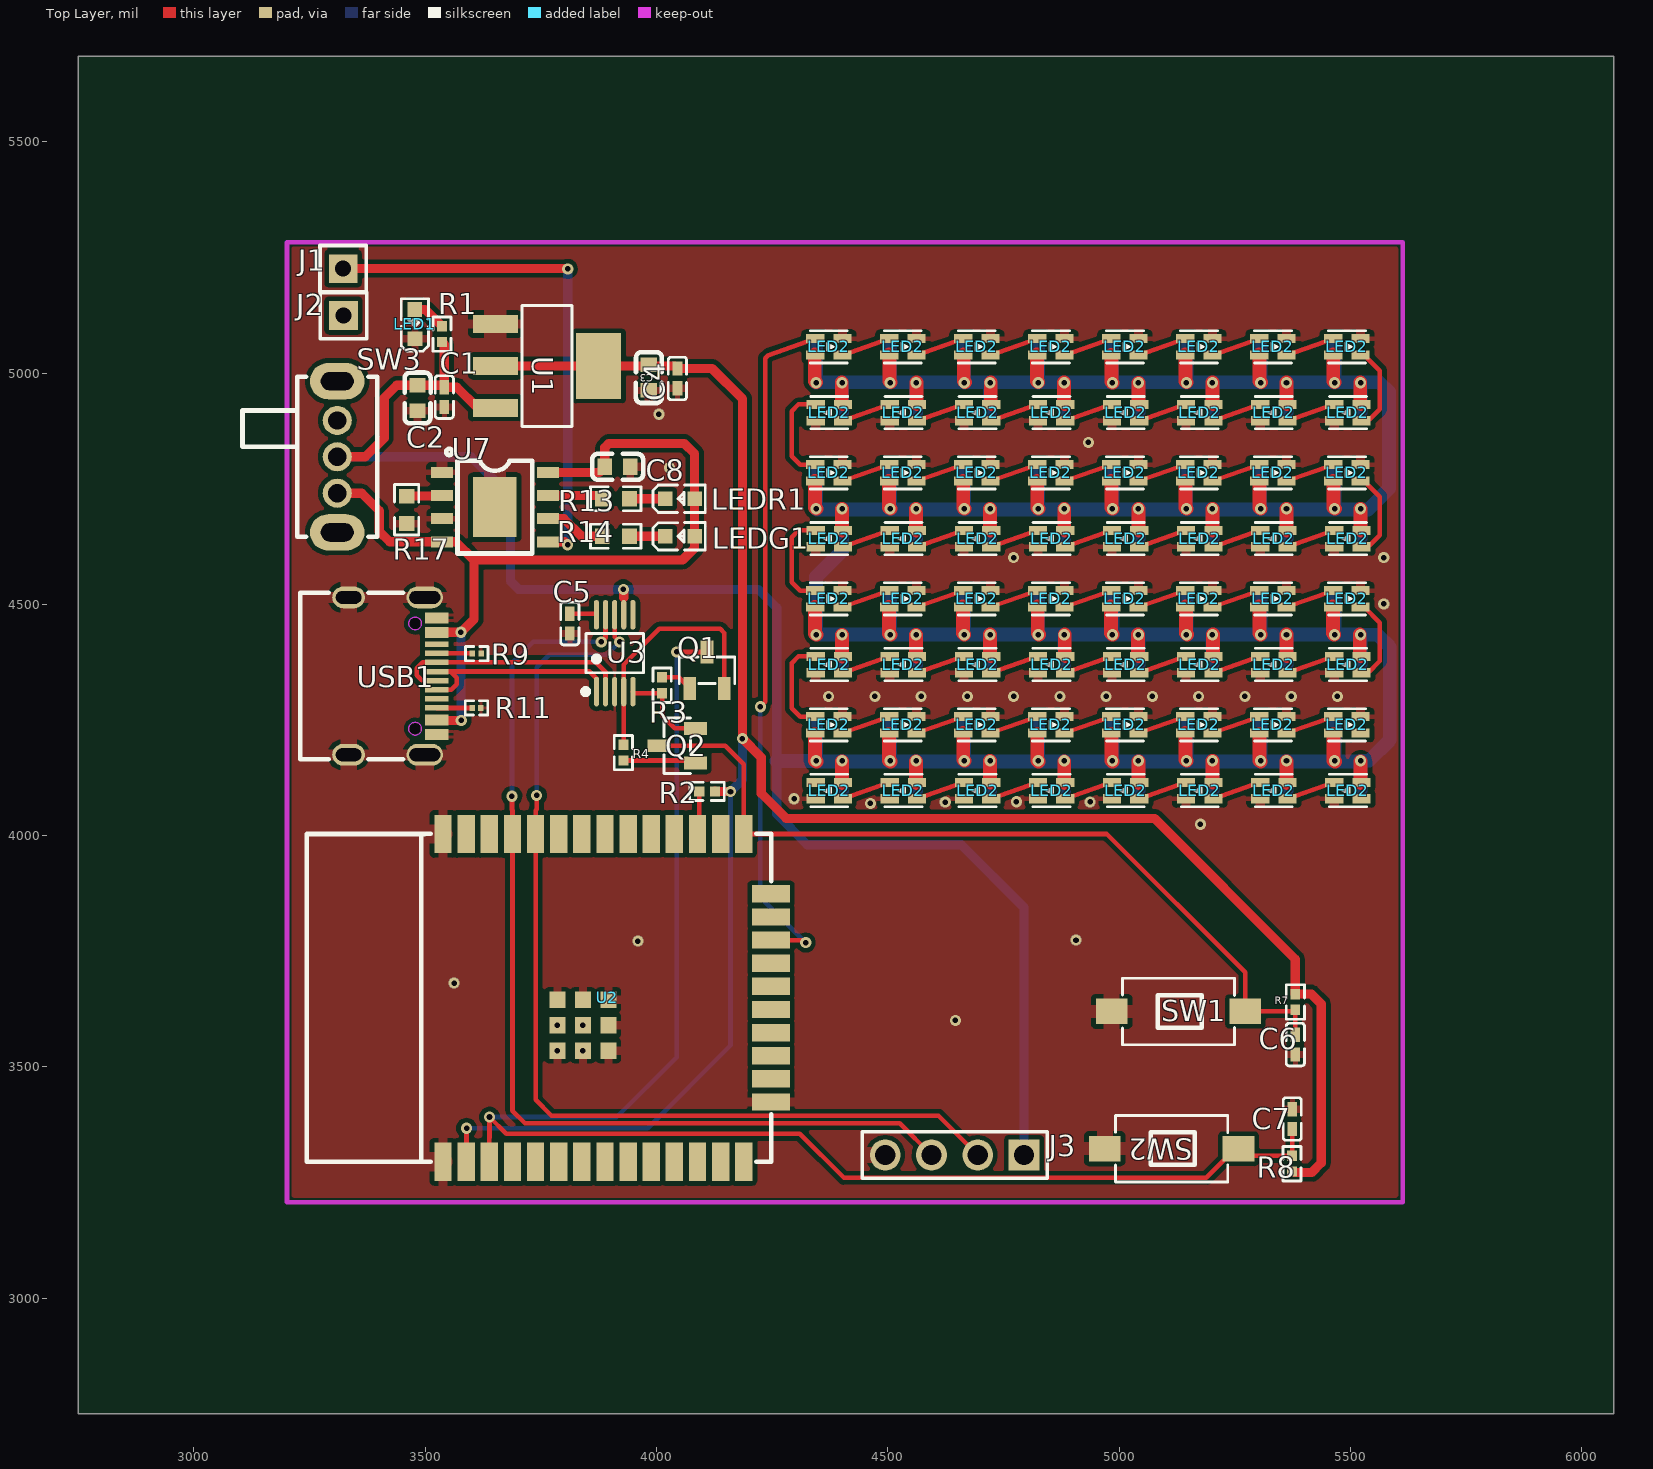
[diagram p0: Top Layer view]
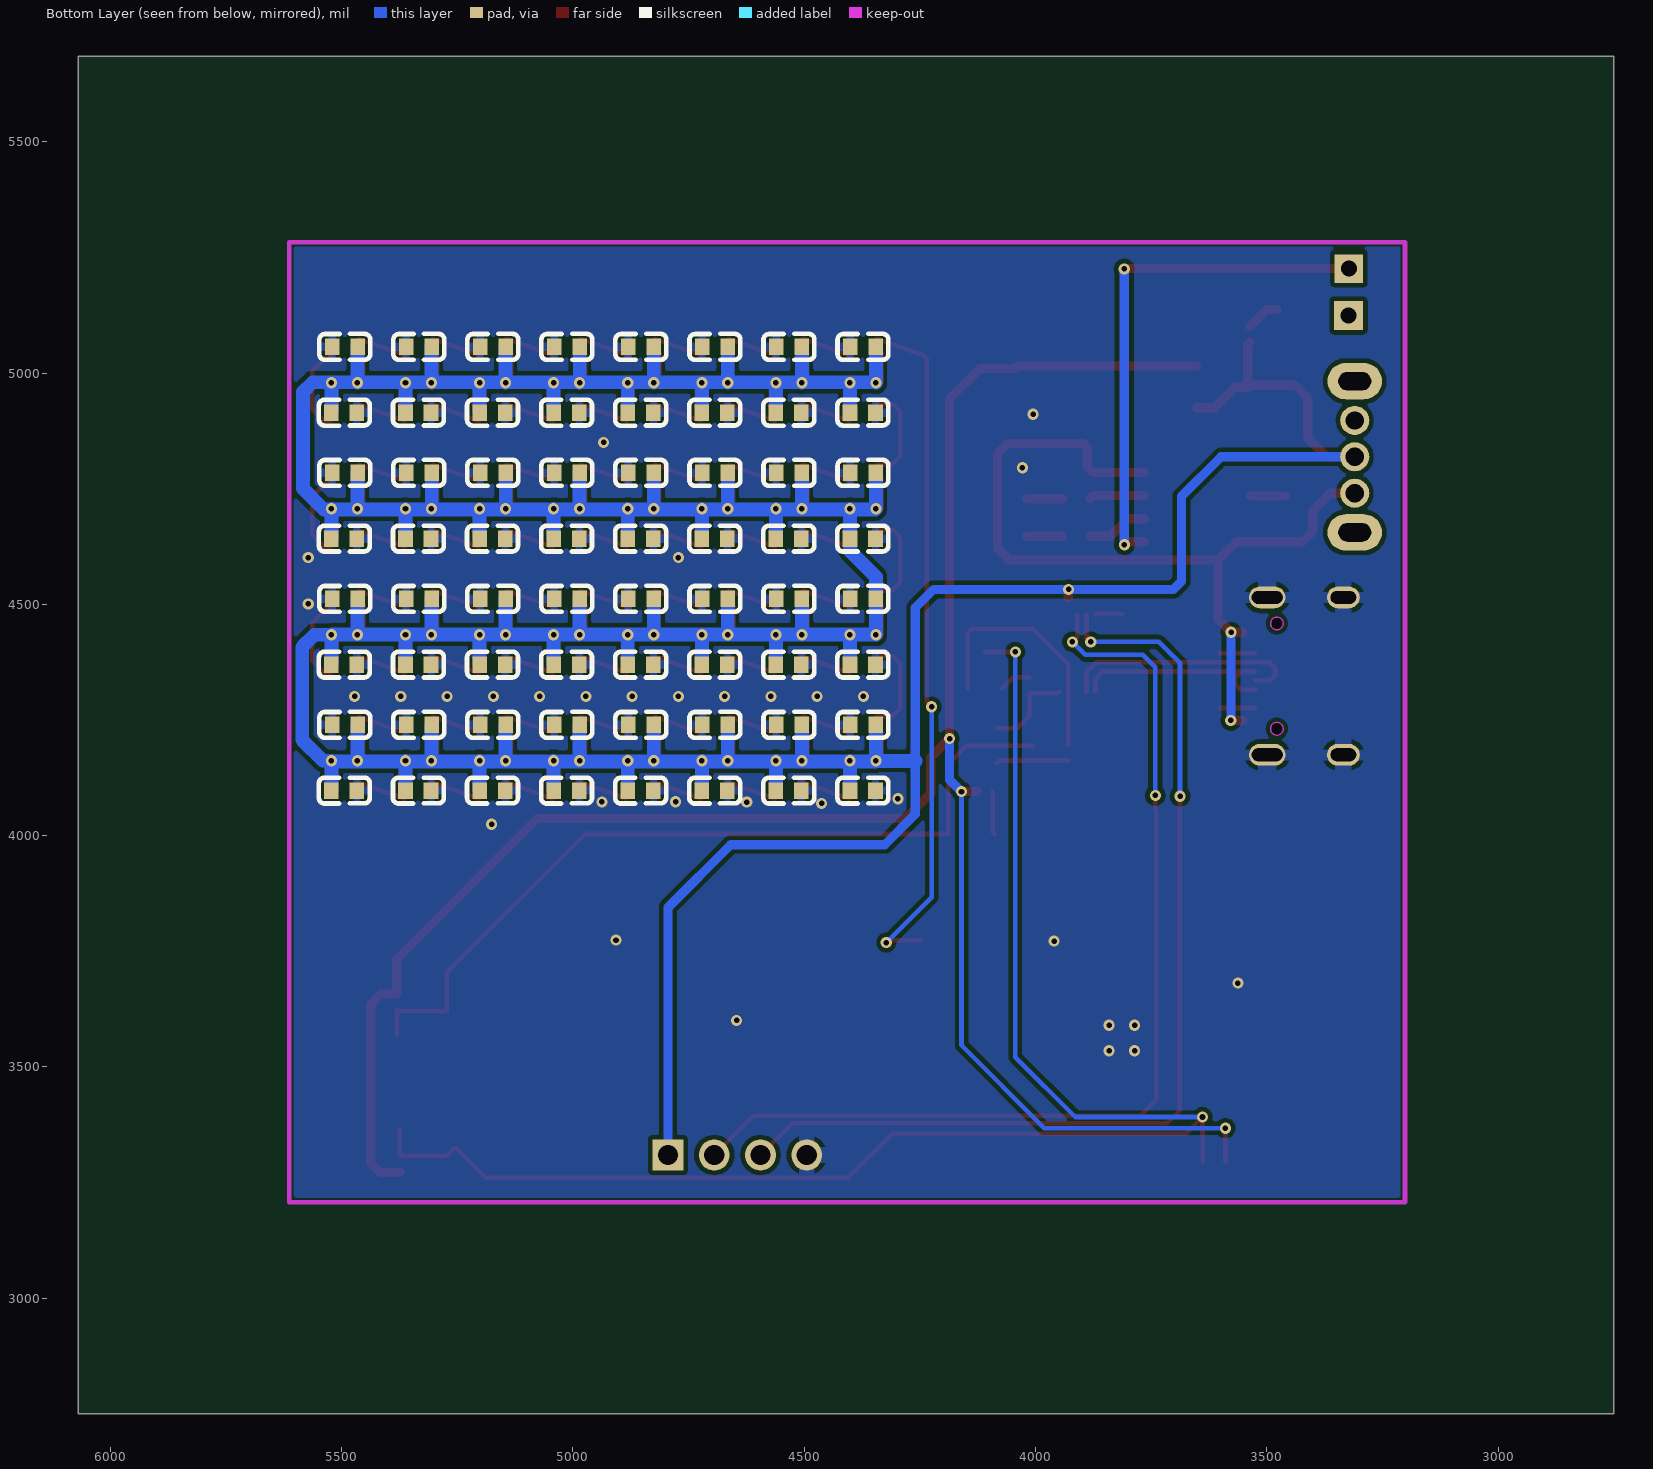
[diagram p1: Bottom Layer view, seen from below]
# Altium PCB MISC52063.pcbdoc
Units mil, origin at the board's own origin, x right, y up, seen from the top; angles counter-clockwise.
Board outline 3318.73 x 2934.56 mil, 2 copper layers (Top Layer, Bottom Layer), stack 62.206 mil thick; 99 components, 49 nets, 539 pads, 112 vias.

## Layer stack, top to bottom
Top Solder Mask Layer: solder mask 0.394, Dk 3.3
Top Layer: signal copper 1.379
Dielectric1: surface 59.449, FR4, Dk 4.5
Bottom Layer: signal copper 1.378
Bottom Solder Mask Layer: solder mask 0.394, Dk 3.3

## Board outline
6068.73,2750 2750,2750 2750,5684.56 6068.73,5684.56

## Design rules (kind name [scope] priority, off if disabled: settings)
BoardOutlineClearance Plane_Default_1 [All] p2 off: genericclearance=5.98 ignorepadtopadclearanceinfootprint=FALSE except(0: Arc-SplitContinuation Track-SplitContinuation SMDPad-SplitContinuation THPad-SplitContinuation Via-SplitContinuation Fill-SplitContinuation Region-SplitContinuation Poly-SplitContinuation Text-SplitContinuation Hole-SplitContinuation; 5.98: Arc-OutlineEdge Track-OutlineEdge SMDPad-OutlineEdge THPad-OutlineEdge Via-OutlineEdge Fill-OutlineEdge Region-OutlineEdge Poly-OutlineEdge Text-OutlineEdge Hole-OutlineEdge Arc-CutoutEdge Track-CutoutEdge SMDPad-CutoutEdge THPad-CutoutEdge Via-CutoutEdge Fill-CutoutEdge Region-CutoutEdge Poly-CutoutEdge Text-CutoutEdge Hole-CutoutEdge)
BoardOutlineClearance Copper_gge30915_1 [All] p4 off: genericclearance=5.98 ignorepadtopadclearanceinfootprint=FALSE except(0: Arc-SplitContinuation Track-SplitContinuation SMDPad-SplitContinuation THPad-SplitContinuation Via-SplitContinuation Fill-SplitContinuation Region-SplitContinuation Poly-SplitContinuation Text-SplitContinuation Hole-SplitContinuation; 5.98: Arc-OutlineEdge Track-OutlineEdge SMDPad-OutlineEdge THPad-OutlineEdge Via-OutlineEdge Fill-OutlineEdge Region-OutlineEdge Text-OutlineEdge Hole-OutlineEdge Arc-CutoutEdge Track-CutoutEdge SMDPad-CutoutEdge THPad-CutoutEdge Via-CutoutEdge Fill-CutoutEdge Region-CutoutEdge Text-CutoutEdge Hole-CutoutEdge; 10: Poly-OutlineEdge Poly-CutoutEdge)
BoardOutlineClearance Copper_gge30960_1 [All] p6 off: genericclearance=5.98 ignorepadtopadclearanceinfootprint=FALSE except(0: Arc-SplitContinuation Track-SplitContinuation SMDPad-SplitContinuation THPad-SplitContinuation Via-SplitContinuation Fill-SplitContinuation Region-SplitContinuation Poly-SplitContinuation Text-SplitContinuation Hole-SplitContinuation; 5.98: Arc-OutlineEdge Track-OutlineEdge SMDPad-OutlineEdge THPad-OutlineEdge Via-OutlineEdge Fill-OutlineEdge Region-OutlineEdge Text-OutlineEdge Hole-OutlineEdge Arc-CutoutEdge Track-CutoutEdge SMDPad-CutoutEdge THPad-CutoutEdge Via-CutoutEdge Fill-CutoutEdge Region-CutoutEdge Text-CutoutEdge Hole-CutoutEdge; 10: Poly-OutlineEdge Poly-CutoutEdge)
BoardOutlineClearance Default_1 [All] p8: genericclearance=5.98 ignorepadtopadclearanceinfootprint=FALSE except(0: Arc-SplitContinuation Track-SplitContinuation SMDPad-SplitContinuation THPad-SplitContinuation Via-SplitContinuation Fill-SplitContinuation Region-SplitContinuation Poly-SplitContinuation Text-SplitContinuation Hole-SplitContinuation; 5.98: Arc-OutlineEdge Track-OutlineEdge SMDPad-OutlineEdge THPad-OutlineEdge Via-OutlineEdge Fill-OutlineEdge Region-OutlineEdge Text-OutlineEdge Hole-OutlineEdge Arc-CutoutEdge Track-CutoutEdge SMDPad-CutoutEdge THPad-CutoutEdge Via-CutoutEdge Fill-CutoutEdge Region-CutoutEdge Text-CutoutEdge Hole-CutoutEdge; 10: Poly-OutlineEdge Poly-CutoutEdge)
Clearance Plane_Default [All] p1 off: gap=5.98 ignorepadtopadclearanceinfootprint=FALSE except(0: Arc-Arc)
Clearance Copper_gge30915 [All] p3 off: gap=5.98 ignorepadtopadclearanceinfootprint=FALSE except(0: Arc-Arc; 10: Poly-Track Poly-SMDPad Poly-THPad Poly-Via Poly-Fill Poly-Region Poly-Poly Poly-Arc Poly-Text Poly-Hole)
Clearance Copper_gge30960 [All] p5 off: gap=5.98 ignorepadtopadclearanceinfootprint=FALSE except(0: Arc-Arc; 10: Poly-Track Poly-SMDPad Poly-THPad Poly-Via Poly-Fill Poly-Region Poly-Poly Poly-Arc Poly-Text Poly-Hole)
Clearance Default [All] p7: gap=5.98 ignorepadtopadclearanceinfootprint=FALSE except(0: Arc-Arc; 10: Poly-Track Poly-SMDPad Poly-THPad Poly-Via Poly-Fill Poly-Region Poly-Poly Poly-Arc Poly-Text Poly-Hole)
DiffPairsRouting differentialPair [All] p1: maxlimit=6 minlimit=6 mostfreqgap=6 toplayer_minwidth=5 toplayer_prefwidth=10 toplayer_maxwidth=100 toplayer_mingap=6 toplayer_prefgap=6 toplayer_maxgap=6 bottomlayer_minwidth=5 bottomlayer_prefwidth=10 bottomlayer_maxwidth=100 bottomlayer_mingap=6 bottomlayer_prefgap=6 bottomlayer_maxgap=6 maxuncoupledlength=10
HoleToHoleClearance otherClearance [All] p1: gap=11.8 allowstackedmicrovias=TRUE
Length netLength [All] p1: minlimit=0 maxlimit=0
PasteMaskExpansion Common [All] p1: expansion=0
PlaneConnect Default_4 [All] p1: planeconnectstyle=Relief reliefexpansion=20 reliefentries=4 reliefconductorwidth=0 reliefairgap=10
PolygonConnect gge30960 [All] p1 off: connectstyle=Relief reliefconductorwidth=0 reliefentries=4 polygonreliefangle="90 Angle" airgapwidth=10 via.connectstyle=Relief via.reliefconductorwidth=10 via.reliefentries=4 via.polygonreliefangle="90 Angle" via.airgapwidth=10
PolygonConnect gge30915 [All] p2: connectstyle=Relief reliefconductorwidth=0 reliefentries=4 polygonreliefangle="90 Angle" airgapwidth=10 via.connectstyle=Relief via.reliefconductorwidth=10 via.reliefentries=4 via.polygonreliefangle="90 Angle" via.airgapwidth=10
RoutingVias Default_3 [All] p1: holewidth=12.01 width=24.02 viastyle="Through Hole" minholewidth=12.01 minwidth=24.02 maxholewidth=2362 maxwidth=3938
SolderMaskExpansion Common_1 [IsVia] p1: expansion=-1000 istentingtop=TRUE
SolderMaskExpansion Common_1 [All] p2: expansion=2 istentingtop=FALSE
Width Default_2 [All] p1: maxlimit=1000 minlimit=10 preferedwidth=10

## Components (designator, comment, footprint, x,y, rotation, side; value= is the part's Value field where it differs from the comment)
C1 "100nF" C0402 3541.1,4947.9 r90 top
C2 "22uF" C0603 3483.26,4945.73 r270 top
C3 "22uF" C0603 3983.19,4989.83 r270 top
C4 "100nF" C0402 4044.95,4988.21 r90 top
C5 "100nF" C0402 3812.38,4458.38 r90 top
C6 "100nF" C0402 5380.55,3548.42 r270 top
C7 "100nF" C0402 5373.94,3387.47 r90 top
C8 "100nF" C0603 3915.51,4797.39 r180 top
J1 "HDR-M-2.54_1x1" HDR-M-2.54_1X1 3322.44,5225.66 r90 top
J2 "HDR-M-2.54_1x1" HDR-M-2.54_1X1 3323.19,5124.2 r90 top
J3 "2.54-1*4" HDR-TH_4P-P2.54-V-M-1 4644.17,3309.76 r180 top
LED1 "XL-1608SURC-06" LED0603-RD_RED 3477.68,5105.77 r90 top
LED2 "WS2812B-0807幻彩" LED-SMD_4P-L2.0-W1.8-TL 5334.08,4097.5 r0 top
LED2 "WS2812B-0807幻彩" LED-SMD_4P-L2.0-W1.8-TL 5494.19,4097.5 r0 top
LED2 "WS2812B-0807幻彩" LED-SMD_4P-L2.0-W1.8-TL 5013.86,4097.5 r0 top
LED2 "WS2812B-0807幻彩" LED-SMD_4P-L2.0-W1.8-TL 5173.97,4097.5 r0 top
LED2 "WS2812B-0807幻彩" LED-SMD_4P-L2.0-W1.8-TL 4693.64,4097.5 r0 top
LED2 "WS2812B-0807幻彩" LED-SMD_4P-L2.0-W1.8-TL 4853.75,4097.5 r0 top
LED2 "WS2812B-0807幻彩" LED-SMD_4P-L2.0-W1.8-TL 4533.53,4097.5 r0 top
LED2 "WS2812B-0807幻彩" LED-SMD_4P-L2.0-W1.8-TL 5012.21,4239.55 r180 top
LED2 "WS2812B-0807幻彩" LED-SMD_4P-L2.0-W1.8-TL 5332.2,4239.55 r180 top
LED2 "WS2812B-0807幻彩" LED-SMD_4P-L2.0-W1.8-TL 4852.21,4239.55 r180 top
LED2 "WS2812B-0807幻彩" LED-SMD_4P-L2.0-W1.8-TL 5492.2,4239.55 r180 top
LED2 "WS2812B-0807幻彩" LED-SMD_4P-L2.0-W1.8-TL 5172.21,4239.55 r180 top
LED2 "WS2812B-0807幻彩" LED-SMD_4P-L2.0-W1.8-TL 4532.21,4239.55 r180 top
LED2 "WS2812B-0807幻彩" LED-SMD_4P-L2.0-W1.8-TL 4692.21,4239.55 r180 top
LED2 "WS2812B-0807幻彩" LED-SMD_4P-L2.0-W1.8-TL 4853.75,4369.81 r0 top
LED2 "WS2812B-0807幻彩" LED-SMD_4P-L2.0-W1.8-TL 4533.53,4369.81 r0 top
LED2 "WS2812B-0807幻彩" LED-SMD_4P-L2.0-W1.8-TL 5494.19,4369.81 r0 top
LED2 "WS2812B-0807幻彩" LED-SMD_4P-L2.0-W1.8-TL 5334.08,4369.81 r0 top
LED2 "WS2812B-0807幻彩" LED-SMD_4P-L2.0-W1.8-TL 5013.86,4369.81 r0 top
LED2 "WS2812B-0807幻彩" LED-SMD_4P-L2.0-W1.8-TL 5173.97,4369.81 r0 top
LED2 "WS2812B-0807幻彩" LED-SMD_4P-L2.0-W1.8-TL 4693.64,4369.81 r0 top
LED2 "WS2812B-0807幻彩" LED-SMD_4P-L2.0-W1.8-TL 5332.2,4784.17 r180 top
LED2 "WS2812B-0807幻彩" LED-SMD_4P-L2.0-W1.8-TL 5012.21,4784.17 r180 top
LED2 "WS2812B-0807幻彩" LED-SMD_4P-L2.0-W1.8-TL 5172.21,4784.17 r180 top
LED2 "WS2812B-0807幻彩" LED-SMD_4P-L2.0-W1.8-TL 4692.21,4784.17 r180 top
LED2 "WS2812B-0807幻彩" LED-SMD_4P-L2.0-W1.8-TL 4532.21,4784.17 r180 top
LED2 "WS2812B-0807幻彩" LED-SMD_4P-L2.0-W1.8-TL 5492.2,4784.17 r180 top
LED2 "WS2812B-0807幻彩" LED-SMD_4P-L2.0-W1.8-TL 4852.21,4784.17 r180 top
LED2 "WS2812B-0807幻彩" LED-SMD_4P-L2.0-W1.8-TL 5494.19,4642.11 r0 top
LED2 "WS2812B-0807幻彩" LED-SMD_4P-L2.0-W1.8-TL 5334.08,4642.11 r0 top
LED2 "WS2812B-0807幻彩" LED-SMD_4P-L2.0-W1.8-TL 4532.21,5056.47 r180 top
LED2 "WS2812B-0807幻彩" LED-SMD_4P-L2.0-W1.8-TL 5332.2,5056.47 r180 top
LED2 "WS2812B-0807幻彩" LED-SMD_4P-L2.0-W1.8-TL 5012.21,5056.47 r180 top
LED2 "WS2812B-0807幻彩" LED-SMD_4P-L2.0-W1.8-TL 5172.21,5056.47 r180 top
LED2 "WS2812B-0807幻彩" LED-SMD_4P-L2.0-W1.8-TL 4692.21,5056.47 r180 top
LED2 "WS2812B-0807幻彩" LED-SMD_4P-L2.0-W1.8-TL 4852.21,5056.47 r180 top
LED2 "WS2812B-0807幻彩" LED-SMD_4P-L2.0-W1.8-TL 5494.19,4914.42 r0 top
LED2 "WS2812B-0807幻彩" LED-SMD_4P-L2.0-W1.8-TL 4533.53,4914.42 r0 top
LED2 "WS2812B-0807幻彩" LED-SMD_4P-L2.0-W1.8-TL 5334.08,4914.42 r0 top
LED2 "WS2812B-0807幻彩" LED-SMD_4P-L2.0-W1.8-TL 4853.75,4914.42 r0 top
LED2 "WS2812B-0807幻彩" LED-SMD_4P-L2.0-W1.8-TL 4693.64,4914.42 r0 top
LED2 "WS2812B-0807幻彩" LED-SMD_4P-L2.0-W1.8-TL 5173.97,4914.42 r0 top
LED2 "WS2812B-0807幻彩" LED-SMD_4P-L2.0-W1.8-TL 5013.86,4914.42 r0 top
LED2 "WS2812B-0807幻彩" LED-SMD_4P-L2.0-W1.8-TL 4853.75,4642.11 r0 top
LED2 "WS2812B-0807幻彩" LED-SMD_4P-L2.0-W1.8-TL 4533.53,4642.11 r0 top
LED2 "WS2812B-0807幻彩" LED-SMD_4P-L2.0-W1.8-TL 5013.86,4642.11 r0 top
LED2 "WS2812B-0807幻彩" LED-SMD_4P-L2.0-W1.8-TL 4693.64,4642.11 r0 top
LED2 "WS2812B-0807幻彩" LED-SMD_4P-L2.0-W1.8-TL 5492.2,4511.86 r180 top
LED2 "WS2812B-0807幻彩" LED-SMD_4P-L2.0-W1.8-TL 5012.21,4511.86 r180 top
LED2 "WS2812B-0807幻彩" LED-SMD_4P-L2.0-W1.8-TL 5332.2,4511.86 r180 top
LED2 "WS2812B-0807幻彩" LED-SMD_4P-L2.0-W1.8-TL 4852.21,4511.86 r180 top
LED2 "WS2812B-0807幻彩" LED-SMD_4P-L2.0-W1.8-TL 5172.21,4511.86 r180 top
LED2 "WS2812B-0807幻彩" LED-SMD_4P-L2.0-W1.8-TL 4532.21,4511.86 r180 top
LED2 "WS2812B-0807幻彩" LED-SMD_4P-L2.0-W1.8-TL 4692.21,4511.86 r180 top
LED2 "WS2812B-0807幻彩" LED-SMD_4P-L2.0-W1.8-TL 5492.2,5056.47 r180 top
LED2 "WS2812B-0807幻彩" LED-SMD_4P-L2.0-W1.8-TL 5173.97,4642.11 r0 top
LED2 "WS2812B-0807幻彩" LED-SMD_4P-L2.0-W1.8-TL 4373.42,4642.11 r0 top
LED2 "WS2812B-0807幻彩" LED-SMD_4P-L2.0-W1.8-TL 4373.42,4369.81 r0 top
LED2 "WS2812B-0807幻彩" LED-SMD_4P-L2.0-W1.8-TL 4373.42,4914.42 r0 top
LED2 "WS2812B-0807幻彩" LED-SMD_4P-L2.0-W1.8-TL 4373.42,4097.5 r0 top
LED2 "WS2812B-0807幻彩" LED-SMD_4P-L2.0-W1.8-TL 4372.21,5056.47 r180 top
LED2 "WS2812B-0807幻彩" LED-SMD_4P-L2.0-W1.8-TL 4372.21,4239.55 r180 top
LED2 "WS2812B-0807幻彩" LED-SMD_4P-L2.0-W1.8-TL 4372.21,4784.17 r180 top
LED2 "WS2812B-0807幻彩" LED-SMD_4P-L2.0-W1.8-TL 4372.21,4511.86 r180 top
LEDG1 "" LED_0603 4052.62,4647.17 r0 top
LEDR1 "" LED_0603 4052.62,4728.32 r0 top
Q1 "SS8050-G" SOT-23-3_L2.9-W1.3-P1.90-LS2.4-BR 4108.98,4357.55 r270 top
Q2 "SS8050-G" SOT-23-3_L2.9-W1.3-P1.90-LS2.4-BR 4044.49,4194.4 r0 top
R1 "2kΩ" R0402 3536.18,5084.08 r270 top
R2 "10kΩ" R0402 4108.98,4095.74 r0 top
R3 "10kΩ" R0402 4011.97,4325.03 r90 top
R4 "10kΩ" R0402 3928.14,4179.47 r270 top
R7 "10kΩ" R0402 5380.55,3640.46 r270 top
R8 "10kΩ" R0402 5373.39,3291.02 r90 top
R9 "5.1kΩ" R0201 3611.31,4393.38 r180 top
R11 "5.1kΩ" R0201 3610.75,4275.98 r0 top
R13 "1K" R0603 3911.86,4728.32 r0 top
R14 "1K" R0603 3911.86,4647.17 r0 top
R17 "1.2K" R0603 3459.69,4704.24 r90 top
SW1 "TSB008A2530A" SW-SMD_L6.0-W3.5-LS8.0 5128.11,3620.07 r0 top
SW2 "TSB008A2530A" SW-SMD_L6.0-W3.5-LS8.0 5113.23,3323.54 r0 top
SW3 "" 拨动开关_侧 3309.76,4818.89 r270 top
U1 "AMS1117-3.3" SOT-223-4_L6.5-W3.5-P2.30-LS7.0-BR 3763.26,5015.18 r180 top
U2 "ESP32-WROOM-32E-N16" WIFI-SMD_ESP32-WROOM-32E 3892.87,3649.29 r0 top
U3 "CH340E" MSOP-10_L3.0-W3.0-P0.50-LS5.0-BL 3909.35,4394.48 r0 top
U7 "TP4056" ESOP-8_L4.9-W3.9-P1.27-LS6.0-BL-EP 3650.42,4710.13 r270 top
USB1 "KH-TYPE-C-16P-T" USB-C-SMD_KH-TYPE-C-16P 3429.41,4344.87 r270 top

## Footprints (in the part's own frame and the unit in brackets; to place one, negate y for a bottom-side part, rotate by r counter-clockwise, add the part's x,y. Pads: shape width x height; smd on the part's side, far side on the other; paste and mask are expansions set on the pad)
C0402 [mm]
  rect 0.79x0.54 smd paste-100 mask+0.051: 1(-0.545,0) 2(0.545,0)
  silkscreen extent -1.17,-0.5 1.17,0.5
C0603 [mm]
  rect 0.8x0.9 smd: 1(-0.7,0) 2(0.7,0)
  silkscreen extent -1.41,-0.71 1.39,0.72
ESOP-8_L4.9-W3.9-P1.27-LS6.0-BL-EP [mm]
  rect 0.6x1.2 smd paste+0 mask+0.051: 1(-1.905,-2.908) 2(-0.635,-2.908) 3(0.635,-2.908) 4(1.905,-2.908) 5(1.905,2.908) 6(0.635,2.908) 7(-0.635,2.908) 8(-1.905,2.908)
  rect 3.3x2.4 smd paste+0 mask+0.051: 9(0,0)
  silkscreen extent -3.2,-2.67 2.55,2.05
HDR-M-2.54_1X1 [mil]
  rect 62x62 hole 35 paste+0 mask+2: 1(0,0)
  silkscreen extent -50,-50 50,50
HDR-TH_4P-P2.54-V-M-1 [mm]
  rect 1.7x1.7 hole 1.1: 1(-3.81,0)
  round 1.7 hole 1.1: 2(-1.27,0) 3(1.27,0) 4(3.81,0)
  silkscreen extent -5.08,-1.27 5.08,1.27
LED0603-RD_RED [mm]
  rect 0.8x0.8 smd: 1(-0.8,-0.003) 2(0.8,0.003)
  silkscreen extent -1.49,-0.75 1.39,0.76
LED-SMD_4P-L2.0-W1.8-TL [mm]
  rect 1x0.5 smd paste+0 mask+0.05: 1(0.75,0.45) 2(-0.75,0.45) 3(-0.75,-0.45) 4(0.75,-0.45)
  rect 0.8x0.9 smd far side: 5(-0.705,-0.003) 6(0.695,-0.003)
  silkscreen extent -1.02,-0.89 1.02,0.89
LED_0603 [mil]
  rect 31.5x31.5 smd paste+0 mask+2: 1(-33.5,-0.4) 2(29.5,-0.2)
  silkscreen extent -61,-30 53,30
MSOP-10_L3.0-W3.0-P0.50-LS5.0-BL [mm]
  oval 0.28x1.62 smd: 1(-1,-2.11) 2(-0.5,-2.11) 3(0,-2.11) 4(0.5,-2.11) 5(1,-2.11) 6(1,2.11) 7(0.5,2.11) 8(0,2.11) 9(-0.5,2.11) 10(-1,2.11)
  silkscreen extent -1.74,-2.26 1.58,1.07
R0201 [mil]
  rect 11.93x12.76 smd paste-3937.01 mask+2: 1(-9.51,0) 2(9.51,0)
  silkscreen extent -24,-15 24,15
R0402 [mm]
  rect 0.566x0.54 smd paste-100 mask+0.051: 1(-0.433,0) 2(0.433,0)
  silkscreen extent -0.94,-0.5 0.94,0.5
R0603 [mil]
  rect 31.75x34.02 smd paste-3937.01 mask+2: 1(-29.66,0) 2(29.66,0)
  silkscreen extent -55,-26 55,26
SOT-23-3_L2.9-W1.3-P1.90-LS2.4-BR [mm]
  rect 1.25x0.7 smd: 1(1,-0.95) 2(1,0.95) 3(-1,0)
  silkscreen extent -0.73,-1.53 0.73,1.53
SOT-223-4_L6.5-W3.5-P2.30-LS7.0-BR [mm]
  rect 2.47x0.98 smd: 1(2.835,-2.3) 2(2.835,0) 3(2.835,2.3)
  rect 2.47x3.6 smd: 4(-2.835,0)
  silkscreen extent -1.37,-3.33 1.37,3.33
SW-SMD_L6.0-W3.5-LS8.0 [mm]
  rect 1.74x1.4 smd: 1(-3.67,0) 2(3.67,0)
  silkscreen extent -3.08,-1.83 3.08,1.83
USB-C-SMD_KH-TYPE-C-16P [mm]
  oval 1.2x2 hole 0.7 slot 1.7 at 90 deg: 1(-4.32,1.765) 2(4.32,1.765)
  oval 1.2x1.8 hole 0.7 slot 1.4 at 90 deg: 3(-4.32,-2.415) 4(4.32,-2.415)
  rect 0.3x1.3 smd paste-100 mask+0.05: A1(-3.35,2.415) A4(-2.55,2.415) A5(-1.25,2.415) A6(-0.25,2.415) A7(0.25,2.415) A8(1.25,2.415) A9(2.55,2.415) A12(3.35,2.415) B1(3.05,2.415) B4(2.25,2.415) B5(1.75,2.415) B6(0.75,2.415) B7(-0.75,2.415) B8(-1.75,2.415) B9(-2.25,2.415) B12(-3.05,2.415)
  Board Outline Layer circle w0.003: c-2.89,1.235 r0.35
  Board Outline Layer circle w0.003: c2.89,1.235 r0.35
  Board Outline Layer region: -2.89,1.585 -2.738,1.55 -2.616,1.453 -2.549,1.313 -2.549,1.157 -2.616,1.017 -2.738,0.92 -2.89,0.885 -2.89,0.885 -3.042,0.92 -3.164,1.017 -3.231,1.157 -3.231,1.313 -3.164,1.453 -3.042,1.55 -2.89,1.585
  Board Outline Layer region: -2.89,1.585 -2.812,1.576 -2.738,1.55 -2.672,1.509 -2.616,1.453 -2.575,1.387 -2.549,1.313 -2.54,1.235 -2.549,1.157 -2.575,1.083 -2.616,1.017 -2.672,0.961 -2.738,0.92 -2.812,0.894 -2.89,0.885 -2.968,0.894 -3.042,0.92 -3.108,0.961 -3.164,1.017 -3.205,1.083 -3.231,1.157 -3.24,1.235 -3.231,1.313 -3.205,1.387 -3.164,1.453 -3.108,1.509 -3.042,1.55 -2.968,1.576
  Board Outline Layer region: 2.89,1.585 3.042,1.55 3.164,1.453 3.231,1.313 3.231,1.157 3.164,1.017 3.042,0.92 2.89,0.885 2.89,0.885 2.738,0.92 2.616,1.017 2.549,1.157 2.549,1.313 2.616,1.453 2.738,1.55 2.89,1.585
  Board Outline Layer region: 2.89,1.585 2.968,1.576 3.042,1.55 3.108,1.509 3.164,1.453 3.205,1.387 3.231,1.313 3.24,1.235 3.231,1.157 3.205,1.083 3.164,1.017 3.108,0.961 3.042,0.92 2.968,0.894 2.89,0.885 2.812,0.894 2.738,0.92 2.672,0.961 2.616,1.017 2.575,1.083 2.549,1.157 2.54,1.235 2.549,1.313 2.575,1.387 2.616,1.453 2.672,1.509 2.738,1.55 2.812,1.576
  Multi-Layer board cut-out: -2.89,1.585 -2.738,1.55 -2.616,1.453 -2.549,1.313 -2.549,1.157 -2.616,1.017 -2.738,0.92 -2.89,0.885 -2.89,0.885 -3.042,0.92 -3.164,1.017 -3.231,1.157 -3.231,1.313 -3.164,1.453 -3.042,1.55 -2.89,1.585
  Multi-Layer board cut-out: 2.89,1.585 3.042,1.55 3.164,1.453 3.231,1.313 3.231,1.157 3.164,1.017 3.042,0.92 2.89,0.885 2.89,0.885 2.738,0.92 2.616,1.017 2.549,1.157 2.549,1.313 2.616,1.453 2.738,1.55 2.89,1.585
  silkscreen extent -4.57,-5.08 4.57,0.57
WIFI-SMD_ESP32-WROOM-32E [mm]
  rect 0.95x2.1 smd: 1(-9.003,-9) 2(-7.733,-9) 3(-6.463,-9) 4(-5.193,-9) 5(-3.923,-9) 6(-2.653,-9) 7(-1.383,-9) 8(-0.113,-9) 9(1.157,-9) 10(2.427,-9) 11(3.697,-9) 12(4.967,-9) 13(6.237,-9) 14(7.507,-9) 25(7.507,9) 26(6.237,9) 27(4.967,9) 28(3.697,9) 29(2.427,9) 30(1.157,9) 31(-0.113,9) 32(-1.383,9) 33(-2.653,9) 34(-3.923,9) 35(-5.193,9) 36(-6.463,9) 37(-7.733,9) 38(-9.003,9)
  rect 2.1x0.95 smd: 15(9.003,-5.715) 16(9.003,-4.445) 17(9.003,-3.175) 18(9.003,-1.905) 19(9.003,-0.635) 20(9.003,0.635) 21(9.003,1.905) 22(9.003,3.175) 23(9.003,4.445) 24(9.003,5.715)
  rect 0.9x0.9 smd: 39(-2.722,-2.9) 39(-2.722,-1.5) 39(-2.722,-0.1) 39(-1.322,-2.9) 39(-1.322,-1.5) 39(-1.322,-0.1) 39(0.078,-2.9) 39(0.078,-1.5) 39(0.078,-0.1)
  silkscreen extent -16.48,-9 9.02,9.02
拨动开关_侧 [mil]
  round 63 hole 39.4 paste+0 mask+2: 1(-78.7,0) 2(0,0) 3(78.7,0)
  oval 78.7x118.1 hole 39.4 slot 70.9 at 90 deg paste+0 mask+2: 4(163.4,0) 5(-163.4,0)
  silkscreen extent -173,-205 173,87

## Via types
v1: diameter 24.02, hole 12, Top Layer to Bottom Layer, 112 vias

## Nets (pads, with @x,y where several pads share a name; then routed paths per layer and width w, separated by ;. In a path a pad name is that pad's centre, name@x,y a point inside that pad or via, vN(x,y) a via of type N, cw(c..) or ccw(c..) an arc to the next point about the centre after c; other vN are vias at no path point)
2: U2.24
3V3: C3.1 C4.2 R2.2 R7.1 R8.1 U1.2 U1.4 U2.2 | length 4718
  Top Layer w10: U2.2 3589.21,3295.73 v1(3589.21,3367.64)
  Top Layer w20: U1.2 U1.4 4039.44,5015.18 C4.2 4119.93,5009.67 4185.59,4944.01 v1(4185.59,4209.84) 4226.38,4169.05 4226.38,4091.34 4280.39,4037.32 5076.3,4037.32 5380.55,3733.06 R7.1 5415.32,3657.5 5436.77,3636.06 5436.77,3292.68 5415.82,3271.73 5375.63,3271.73 R8.1 ; R2.2 4126.56,4095.19 v1(4159.68,4095.19)
  Bottom Layer w10: v1(3589.21,3367.64) 3980.55,3367.64 4159.68,3546.77 v1(4159.68,4095.19)
  Bottom Layer w20: v1(4159.68,4095.19) 4185.59,4121.1 v1(4185.59,4209.84)
4: U2.26
5: U2.29
12: U2.14
13: U2.16
14: U2.13
15: U2.23
17: U2.28
18: U2.30
19: U2.31
21: U2.33
22: U2.36
23: U2.37
25: U2.10
26: U2.11
27: U2.12
32: U2.8
33: U2.9
34: U2.6
35: U2.7
$1N3: C5.2 U3.10 | length 58.6
  Top Layer w10: C5.2 3867.69,4479.84 U3.10
$1N5: Q1.2 R4.1 U3.4 | length 546.6
  Top Layer w10: R4.1 3929.04,4197.41 U3.4 3929.04,4369.97 4005.91,4446.84 4137.64,4446.84 4146.38,4438.1 Q1.2
$1N10: R2.1 U2.27 | length 93.6
  Top Layer w10: U2.27 4091.94,4007.13 R2.1
$1N31: R9.2 USB1.A5 | length 77.6
  Top Layer w10: USB1.A5 3601.09,4394.08 R9.2
$1N32: R11.1 USB1.B5 | length 76.7
  Top Layer w10: USB1.B5 R11.1
$1N1136: Q1.1 R3.2 | length 69.5
  Top Layer w10: R3.2 4047.69,4342.07 Q1.1
$1N1137: Q2.1 R4.2 | length 158
  Top Layer w10: R4.2 4078.43,4162.43 Q2.1
$1N19734: LED1.2 R1.1 | length 73.6
  Top Layer w20: LED1.2 3500.05,5137.25 R1.1
$1N23672: Q2.2 R3.1 U3.5 | length 196.6
  Top Layer w10: U3.5 3952.14,4307.99 R3.1 4011.97,4259.44 4039.61,4231.8 Q2.2
$1N26569: R14.1 U7.6 | length 133
  Top Layer w20: U7.6 3799.59,4685.13 3837.55,4647.17 R14.1
$1N26570: R13.1 U7.7 | length 120.1
  Top Layer w20: U7.7 3875.39,4735.13 R13.1
$1N26571: LEDG1.1 R14.2 | length 77.8
  Top Layer w20: R14.2 4018.72,4647.17 LEDG1.1
$1N26572: LEDR1.1 R13.2 | length 77.8
  Top Layer w20: R13.2 4018.72,4728.32 LEDR1.1
$1N26577: R17.2 U7.2 | length 76.7
  Top Layer w20: R17.2 3534.7,4733.9 U7.2
+5V: C1.2 C2.1 J3.1 R1.2 SW3.2 U1.3 U3.7 | length 3386.1
  Top Layer w20: SW3.2 3370.39,4818.89 3411.18,4859.68 3411.18,4946.22 3438.26,4973.29 C2.1 3537.17,4973.29 C1.2 ; R1.2 3541.1,5062.11 C1.2 ; U1.3 3613,4924.63 3568.27,4969.36 C1.2 ; v1(3928.19,4532.28) 3929.04,4531.43 3929.04,4514.65
  Bottom Layer w20: SW3.2 3598.59,4818.89 3684.01,4733.46 3684.01,4549.92 3701.65,4532.28 v1(3928.19,4532.28) 4219.76,4532.28 4259.45,4492.6 4259.45,4046.69 4325.59,3980.55 4658.5,3980.55 4794.17,3844.88 J3.1
B+: J1.1 U7.5 | length 1127.6
  Top Layer w20: J1.1 3807.48,5225.66 v1(3808.03,5225.11) ; U7.5 3801.09,4635.13 v1(3807.48,4628.74)
  Bottom Layer w20: v1(3807.48,4628.74) 3808.03,4629.29 v1(3808.03,5225.11)
B-: J2.1
BOOT: C6.1 Q2.3 R7.2 SW1.2 U2.25 | length 1805.7
  Top Layer w10: Q2.3 4148.11,4194.4 4188.44,4154.08 U2.25 4973.3,4003.63 5272.6,3704.32 SW1.2 5377.2,3620.07 R7.2 C6.1
D+: U3.1 USB1.A6 USB1.B6 | length 461.9
  Top Layer w10: USB1.B6 3556.38,4315.34 3568.27,4327.24 3568.27,4341.57 3555.12,4354.71 ; USB1.A6 3555.12,4354.71 ; U3.1 3869.98,4340.25 3855.51,4354.71 3555.12,4354.71
D-: U3.2 USB1.A7 USB1.B7 | length 526.5
  Top Layer w10: USB1.A7 3523.38,4336.15 3492.43,4336.15 3481.73,4346.85 3481.73,4361.64 3494.49,4374.4 USB1.B7 3868.9,4374.4 3889.67,4353.63 U3.2
EN: C7.1 Q1.3 R8.2 SW2.2 U2.3 | length 3376.4
  Top Layer w10: U2.3 3638.44,3346.3 3638.82,3346.68 v1(3638.82,3391.89) 3674.64,3356.06 4309.6,3356.06 4404.96,3260.71 5188.2,3260.71 5251.02,3323.54 SW2.2 5273.2,3308.06 R8.2 5373.94,3308.61 C7.1 ; v1(4043.38,4397.24) 4043.7,4396.92 Q1.3
  Bottom Layer w10: v1(3638.82,3391.89) 3913.86,3391.89 4043.38,3521.42 v1(4043.38,4397.24)
GND: C1.1 C2.2 C3.2 C4.1 C5.1 C6.2 C7.2 C8.1 J3.4 LED1.1 LED2.3 LED2.5 R9.1 R11.2 R17.1 SW1.1 SW2.1 U1.1 U2.1 U2.15 U2.38 U2.39 U3.3 U7.1 U7.3 U7.9 USB1.1 USB1.2 USB1.3 USB1.4 USB1.A1 USB1.A12 USB1.B1 USB1.B12
  other v1: 3785.72,3535.12 3840.84,3535.12 3785.72,3590.24 3840.84,3590.23 4645.82,3600.79 3562.2,3681.26 3959.6,3772.2 4906.53,3774.41 5175.51,4024.64 4462.01,4069.67 4623.78,4072.6 4777.71,4073.24 4936.85,4073.15 4297.29,4079.78 4371.63,4300.9 4471.63,4300.9 4571.63,4300.9 4671.63,4300.9 4771.63,4300.9 4871.63,4300.9 4971.63,4300.9 5071.63,4300.9 5171.63,4300.9 5271.63,4300.9 5371.63,4300.9 5471.63,4300.9 5571.63,4500.9 4771.63,4600.9 5571.63,4600.9 4027.95,4795.19 4933.2,4850 4004.8,4910.94
POW: C8.2 LEDG1.2 LEDR1.2 SW3.3 U7.4 U7.8 USB1.A4 USB1.A9 USB1.B4 USB1.B9 | length 1859.6
  Top Layer w20: SW3.3 3362.56,4740.19 3400.71,4702.04 3400.71,4657.4 3422.98,4635.13 U7.4 3565.73,4635.13 3605.2,4595.67 ; 3551.18,4439.68 v1(3577.09,4439.68) 3605.2,4467.79 3605.2,4595.67 ; 3551.73,4248.97 v1(3577.64,4248.97) ; U7.8 3875.69,4785.13 C8.2 3887.95,4838.74 3896.77,4847.56 4059.92,4847.56 4082.12,4825.35 LEDR1.2 LEDG1.2 4082.12,4621.73 4056.06,4595.67 3605.2,4595.67
  Bottom Layer w20: v1(3577.09,4439.68) 3577.09,4249.53 v1(3577.64,4248.97)
RXD0: J3.2 U2.34 U3.8 | length 2205.9
  Top Layer w10: v1(3740.79,4086.92) 3740.79,4057.32 3738.44,4054.97 U2.34 3738.44,3428.96 3772.78,3394.61 4609.32,3394.61 J3.2 ; U3.8 3909.35,4429.31 v1(3919.92,4418.73)
  Bottom Layer w10: v1(3740.79,4086.92) 3740.79,4363.61 3767.8,4390.62 3891.81,4390.62 v1(3919.92,4418.73)
TXD0: J3.3 U2.35 U3.9 | length 2187.5
  Top Layer w10: v1(3687.32,4085.27) 3687.32,4056.08 3688.44,4054.97 U2.35 3688.44,3405.65 3715.46,3378.63 4525.3,3378.63 J3.3 ; v1(3880.24,4418.73) 3889.67,4428.16 U3.9
  Bottom Layer w10: v1(3687.32,4085.27) 3687.32,4372.43 3733.62,4418.73 v1(3880.24,4418.73)
VCC: LED2.1 LED2.6 | length 13681.1
  Top Layer w30: LED2.1@4341.88,5039.92 4341.88,4982.77 v1@4344.65,4980 ; LED2.1@4342.46,4219.92 4342.46,4162.77 v1@4345.23,4160 ; LED2.1@4342.46,4494.15 4342.46,4437 v1@4345.23,4434.23 ; LED2.1@4342.46,4766.46 4342.46,4709.3 v1@4345.23,4706.54 ; v1@4400.21,4980 4400.21,4935.44 LED2.1@4402.37,4933.28 ; v1@4400.79,4160 4400.79,4115.44 LED2.1@4402.95,4113.28 ; v1(4400.79,4434.23) 4400.79,4389.67 LED2.1@4402.95,4387.52 ; v1(4400.79,4706.54) 4400.79,4661.98 LED2.1@4402.95,4659.82 ; LED2.1@4502.57,4219.92 4502.57,4162.77 v1@4505.34,4160 ; LED2.1@4502.57,4494.15 4502.57,4437 v1@4505.34,4434.23 ; LED2.1@4502.57,4766.46 4502.57,4709.3 v1@4505.34,4706.54 ; LED2.1@4503.03,5039.92 4503.03,4982.77 v1@4505.8,4980 ; v1@4560.9,4160 4560.9,4115.44 LED2.1@4563.06,4113.28 ; v1(4560.9,4434.23) 4560.9,4389.67 LED2.1@4563.06,4387.52 ; v1(4560.9,4706.54) 4560.9,4661.98 LED2.1@4563.06,4659.82 ; v1@4561.36,4980 4561.36,4935.44 LED2.1@4563.51,4933.28 ; LED2.1@4662.22,4494.92 4662.22,4437.77 v1@4664.99,4435 ; LED2.1@4662.68,4221.84 4662.68,4164.69 v1@4665.45,4161.92 ; LED2.1@4662.68,4766.46 4662.68,4709.3 v1@4665.45,4706.54 ; LED2.1@4663.78,5039.92 4663.78,4982.77 v1@4666.55,4980 ; v1@4720.55,4435 4720.55,4390.44 LED2.1@4722.71,4388.28 ; v1(4721.01,4161.92) 4721.01,4117.36 LED2.1@4723.17,4115.21 ; v1(4721.01,4706.54) 4721.01,4661.98 LED2.1@4723.17,4659.82 ; v1@4722.11,4980 4722.11,4935.44 LED2.1@4724.27,4933.28 ; LED2.1@4822.2,5039.92 4822.2,4982.77 v1@4824.97,4980 ; LED2.1@4822.79,4219.92 4822.79,4162.77 v1@4825.56,4160 ; LED2.1@4822.79,4766.46 4822.79,4709.3 v1@4825.56,4706.54 ; LED2.1@4823.76,4494.92 4823.76,4437.77 v1@4826.53,4435 ; v1@4880.53,4980 4880.53,4935.44 LED2.1@4882.69,4933.28 ; v1@4881.12,4160 4881.12,4115.44 LED2.1@4883.28,4113.28 ; v1(4881.12,4706.54) 4881.12,4661.98 LED2.1@4883.28,4659.82 ; v1@4882.09,4435 4882.09,4390.44 LED2.1@4884.25,4388.28 ; LED2.1@4982.44,4494.92 4982.44,4437.77 v1@4985.2,4435 ; LED2.1@4982.9,4219.92 4982.9,4162.77 v1@4985.67,4160 ; LED2.1@4982.9,4766.46 4982.9,4709.3 v1@4985.67,4706.54 ; LED2.1@4982.9,5038.76 4982.9,4981.61 v1@4985.67,4978.85 ; v1@5040.76,4435 5040.76,4390.44 LED2.1@5042.92,4388.28 ; v1@5041.23,4160 5041.23,4115.44 LED2.1@5043.39,4113.28 ; v1(5041.23,4706.54) 5041.23,4661.98 LED2.1@5043.39,4659.82 ; v1(5041.23,4978.85) 5041.23,4934.29 LED2.1@5043.39,4932.13 ; LED2.1@5142.93,5039.92 5142.93,4982.77 v1@5145.7,4980 ; LED2.1@5143.01,4221.84 5143.01,4164.69 v1@5145.78,4161.92 ; LED2.1@5143.01,4766.46 5143.01,4709.3 v1@5145.78,4706.54 ; LED2.1@5144.23,4494.92 5144.23,4437.77 v1@5147,4435 ; v1@5201.26,4980 5201.26,4935.44 LED2.1@5203.42,4933.28 ; v1(5201.34,4161.92) 5201.34,4117.36 LED2.1@5203.5,4115.21 ; v1(5201.34,4706.54) 5201.34,4661.98 LED2.1@5203.5,4659.82 ; v1@5202.56,4435 5202.56,4390.44 LED2.1@5204.72,4388.28 ; LED2.1@5302.91,4494.92 5302.91,4437.77 v1@5305.67,4435 ; LED2.1@5303.12,4219.92 5303.12,4162.77 v1@5305.89,4160 ; LED2.1@5303.12,4766.46 5303.12,4709.3 v1@5305.89,4706.54 ; LED2.1@5303.3,5039.92 5303.3,4982.77 v1@5306.06,4980 ; v1@5361.24,4435 5361.24,4390.44 LED2.1@5363.39,4388.28 ; v1@5361.45,4160 5361.45,4115.44 LED2.1@5363.61,4113.28 ; v1(5361.45,4706.54) 5361.45,4661.98 LED2.1@5363.61,4659.82 ; v1@5361.63,4980 5361.63,4935.44 LED2.1@5363.78,4933.28 ; LED2.1@5461.58,4494.92 5461.58,4437.77 v1@5464.35,4435 ; LED2.1@5462.49,5039.92 5462.49,4982.77 v1@5465.26,4980 ; LED2.1@5463.23,4219.92 5463.23,4162.77 v1@5466,4160 ; LED2.1@5463.23,4766.46 5463.23,4709.3 v1@5466,4706.54 ; v1@5519.91,4435 5519.91,4390.44 LED2.1@5522.07,4388.28 ; v1@5520.82,4980 5520.82,4935.44 LED2.1@5522.98,4933.28 ; v1@5521.56,4160 5521.56,4115.44 LED2.1@5523.72,4113.28 ; v1(5521.56,4706.54) 5521.56,4661.98 LED2.1@5523.72,4659.82
  Bottom Layer w30: 4259.45,4161.61 4345.1,4161.61 v1@4346.71,4160 ; LED2.6@4344.79,4239.6 v1(4344.79,4161.92) v1@4346.71,4160 ; v1(4344.79,4434.23) v1@4344.79,4435 ; LED2.6@4344.79,4511.91 v1@4344.79,4435 ; LED2.6@4344.79,4784.22 v1(4344.79,4706.54) 4346.32,4705 v1@4400.79,4705 ; v1(4344.79,4978.85) v1@4344.79,4980 ; LED2.6@4344.79,5056.53 v1@4344.79,4980 ; LED2.6@4344.84,4511.97 4344.84,4559.12 4400.79,4615.07 4400.79,4642.01 v1@4400.79,4705 ; LED2.6@4400.79,4097.39 v1@4400.79,4160 ; v1(4400.79,4161.92) v1@4400.79,4160 ; LED2.6@4400.79,4369.7 v1(4400.79,4434.23) ; v1(4400.79,4706.54) v1@4400.79,4705 ; LED2.6@4400.79,4914.31 v1(4400.79,4978.85) ; v1(4504.79,4434.23) v1@4504.79,4435 ; LED2.6@4504.79,4511.91 v1@4504.79,4435 ; v1(4504.79,4706.54) LED2.6@4504.79,4784.22 ; v1(4504.79,4978.85) v1@4504.79,4980 ; LED2.6@4504.79,5056.53 v1@4504.79,4980 ; 4504.84,4178.36 LED2.6@4504.84,4239.66 ; LED2.6@4560.9,4097.39 v1@4560.9,4160 ; v1(4560.9,4161.92) v1@4560.9,4160 ; LED2.6@4560.9,4369.7 v1(4560.9,4434.23) ; LED2.6@4560.9,4642.01 v1@4560.9,4705 ; v1(4560.9,4706.54) v1@4560.9,4705 ; LED2.6@4560.9,4914.31 v1(4560.9,4978.85) ; LED2.6@4664.84,4239.66 4665.01,4239.49 v1(4665.01,4161.92) ; LED2.6@4664.84,4511.97 4665.01,4511.8 v1@4665.01,4435 ; LED2.6@4664.84,4784.27 4665.01,4784.1 v1(4665.01,4706.54) ; LED2.6@4664.84,5056.58 v1@4664.84,4980 ; v1(4665.01,4434.23) v1@4665.01,4435 ; v1(4665.01,4978.85) 4664.84,4979.01 v1@4664.84,4980 ; LED2.6@4721.01,4097.39 v1@4721.01,4160 ; v1(4721.01,4161.92) v1@4721.01,4160 ; LED2.6@4721.01,4369.7 v1(4721.01,4434.23) ; LED2.6@4721.01,4642.01 v1@4721.01,4705 ; v1(4721.01,4706.54) v1@4721.01,4705 ; LED2.6@4721.01,4914.31 v1(4721.01,4978.85) ; LED2.6@4824.84,4239.66 4824.84,4162.09 v1(4825.01,4161.92) ; LED2.6@4824.84,4511.97 4825.01,4511.8 v1@4825.01,4435 ; LED2.6@4824.84,4784.27 4825.01,4784.1 v1(4825.01,4706.54) ; LED2.6@4824.84,5056.58 4825.01,5056.41 v1@4825.01,4980 ; v1(4825.01,4434.23) v1@4825.01,4435 ; v1(4825.01,4978.85) v1@4825.01,4980 ; LED2.6@4881.12,4097.39 v1@4881.12,4160 ; v1(4881.12,4161.92) v1@4881.12,4160 ; LED2.6@4881.12,4369.7 v1(4881.12,4434.23) ; LED2.6@4881.12,4642.01 v1@4881.12,4705 ; v1(4881.12,4706.54) v1@4881.12,4705 ; LED2.6@4881.12,4914.31 v1(4881.12,4978.85) ; LED2.6@4984.84,4239.66 4985.23,4239.27 v1(4985.23,4161.92) ; LED2.6@4984.84,4511.97 4985.23,4511.58 v1@4985.23,4435 ; LED2.6@4984.84,4784.27 4985.23,4783.88 v1(4985.23,4706.54) ; LED2.6@4984.84,5056.58 v1@4984.84,4980 ; v1(4985.23,4434.23) v1@4985.23,4435 ; v1(4985.23,4978.85) 4984.84,4979.23 v1@4984.84,4980 ; LED2.6@5041.23,4097.39 v1@5041.23,4160 ; v1(5041.23,4161.92) v1@5041.23,4160 ; LED2.6@5041.23,4369.7 v1(5041.23,4434.23) ; LED2.6@5041.23,4642.01 v1@5041.23,4705 ; v1(5041.23,4706.54) v1@5041.23,4705 ; LED2.6@5041.23,4914.31 v1(5041.23,4978.85) ; LED2.6@5144.84,4239.66 5145.23,4239.27 v1(5145.23,4161.92) ; LED2.6@5144.84,4511.97 5145.23,4511.58 v1@5145.23,4435 ; LED2.6@5144.84,4784.27 5144.84,4706.93 v1(5145.23,4706.54) ; LED2.6@5144.84,5056.58 5145.23,5056.19 v1@5145.23,4980 ; v1(5145.23,4434.23) v1@5145.23,4435 ; v1(5145.23,4978.85) v1@5145.23,4980 ; LED2.6@5201.34,4097.39 v1@5201.34,4160 ; v1(5201.34,4161.92) v1@5201.34,4160 ; LED2.6@5201.34,4369.7 v1(5201.34,4434.23) ; LED2.6@5201.34,4642.01 v1@5201.34,4705 ; v1(5201.34,4706.54) v1@5201.34,4705 ; LED2.6@5201.34,4914.31 v1(5201.34,4978.85) ; LED2.6@5304.84,4239.66 5305.45,4239.05 v1(5305.45,4161.92) ; LED2.6@5304.84,4511.97 5305.45,4511.36 v1@5305.45,4435 ; LED2.6@5304.84,4784.27 5304.84,4707.15 v1(5305.45,4706.54) ; LED2.6@5304.84,5056.58 5305.45,5055.97 v1@5305.45,4980 ; v1(5305.45,4434.23) v1@5305.45,4435 ; v1(5305.45,4978.85) v1@5305.45,4980 ; LED2.6@5361.45,4097.39 v1@5361.45,4160 ; v1(5361.45,4161.92) v1@5361.45,4160 ; LED2.6@5361.45,4369.7 v1(5361.45,4434.23) ; LED2.6@5361.45,4642.01 v1@5361.45,4705 ; v1(5361.45,4706.54) v1@5361.45,4705 ; LED2.6@5361.45,4914.31 v1(5361.45,4978.85) ; LED2.6@5464.84,4239.66 5464.84,4162.53 v1(5465.45,4161.92) ; LED2.6@5464.84,4511.97 5465.45,4511.36 v1@5465.45,4435 ; LED2.6@5464.84,4784.27 5465.45,4783.66 v1(5465.45,4706.54) ; LED2.6@5464.84,5056.58 v1@5464.84,4980 ; v1(5465.45,4434.23) v1@5465.45,4435 ; v1(5465.45,4978.85) 5464.84,4979.46 v1@5464.84,4980 ; LED2.6@5521.56,4097.39 5521.56,4160 v1@5361.45,4160 ; v1(5521.56,4161.92) 5539.45,4161.92 5584.74,4207.21 5584.74,4407.29 5557.79,4434.23 v1(5521.56,4434.23) ; LED2.6@5521.56,4369.7 v1(5521.56,4434.23) ; LED2.6@5521.56,4642.01 v1@5521.56,4705 ; v1(5521.56,4706.54) v1@5521.56,4705 ; LED2.6@5521.56,4914.31 v1(5521.56,4978.85) ; v1@4344.79,4435 v1@4504.79,4435 ; v1@4344.79,4980 v1@4504.79,4980 ; v1@4346.71,4160 v1@4400.79,4160 ; v1@4400.79,4160 v1@4560.9,4160 ; v1@4400.79,4705 v1@4560.9,4705 ; v1@4504.79,4435 v1@4665.01,4435 ; v1@4504.79,4980 v1@4664.84,4980 ; v1@4560.9,4160 v1@4721.01,4160 ; v1@4560.9,4705 v1@4721.01,4705 ; v1@4664.84,4980 v1@4825.01,4980 ; v1@4665.01,4435 v1@4825.01,4435 ; v1@4721.01,4160 v1@4881.12,4160 ; v1@4721.01,4705 v1@4881.12,4705 ; v1@4825.01,4435 v1@4985.23,4435 ; v1@4825.01,4980 v1@4984.84,4980 ; v1@4881.12,4160 v1@5041.23,4160 ; v1@4881.12,4705 v1@5041.23,4705 ; v1@4984.84,4980 v1@5145.23,4980 ; v1@4985.23,4435 v1@5145.23,4435 ; v1@5041.23,4160 v1@5201.34,4160 ; v1@5041.23,4705 v1@5201.34,4705 ; v1@5145.23,4435 v1@5305.45,4435 ; v1@5145.23,4980 v1@5305.45,4980 ; v1@5201.34,4160 v1@5361.45,4160 ; v1@5201.34,4705 v1@5361.45,4705 ; v1@5305.45,4435 v1@5465.45,4435 ; v1@5305.45,4980 v1@5464.84,4980 ; v1@5361.45,4705 v1@5521.56,4705 ; v1@5464.84,4980 5561.99,4980 5583.2,4958.79 5583.2,4750 5538.2,4705 v1@5521.56,4705 ; v1@5465.45,4435 5520.79,4435 v1(5521.56,4434.23)
  other v1: 4504.79,4161.92
VN: U2.5
VP: U2.4
pads on no net: LED2.2 LED2.4 SW3.1 SW3.4 SW3.5 U2.17 U2.18 U2.19 U2.20 U2.21 U2.22 U2.32 U3.6 USB1.A8 USB1.B8
copper on no net: | length 8700.9
  Top Layer w10: v1(4224.17,4278.74) 4234.66,4289.23 4234.66,5031.69 4241.73,5038.76 4342.68,5074.18 ; 4247.3,3774.3 4316.88,3774.3 v1(4322.28,3768.9) ; 4342.68,4257.26 4310.46,4257.26 4292.22,4275.51 4292.22,4373.06 4306.67,4387.52 4343.9,4387.52 ; 4342.68,4529.57 4310.46,4529.57 4292.22,4547.81 4292.22,4645.37 4306.67,4659.82 4343.9,4659.82 ; 4342.68,4801.88 4310.46,4801.88 4292.22,4820.12 4292.22,4917.68 4306.67,4932.13 4343.9,4932.13 ; 4401.73,4221.84 4502.68,4257.26 ; 4401.73,4494.15 4502.68,4529.57 ; 4401.73,4766.46 4502.68,4801.88 ; 4401.73,5038.76 4502.68,5074.18 ; 4402.95,4079.79 4504.01,4115.21 ; 4402.95,4352.1 4504.01,4387.52 ; 4402.95,4624.4 4504.01,4659.82 ; 4402.95,4896.71 4504.01,4932.13 ; 4561.73,4221.84 4662.68,4257.26 ; 4561.73,4494.15 4662.68,4529.57 ; 4561.73,4766.46 4662.68,4801.88 ; 4561.73,5038.76 4662.68,5074.18 ; 4563.06,4079.79 4664.12,4115.21 ; 4563.06,4352.1 4664.12,4387.52 ; 4563.06,4624.4 4664.12,4659.82 ; 4563.06,4896.71 4664.12,4932.13 ; 4721.73,4221.84 4822.68,4257.26 ; 4721.73,4494.15 4822.68,4529.57 ; 4721.73,4766.46 4822.68,4801.88 ; 4721.73,5038.76 4822.68,5074.18 ; 4723.17,4079.79 4824.23,4115.21 ; 4723.17,4352.1 4824.23,4387.52 ; 4723.17,4624.4 4824.23,4659.82 ; 4723.17,4896.71 4824.23,4932.13 ; 4881.73,4221.84 4982.68,4257.26 ; 4881.73,4494.15 4982.68,4529.57 ; 4881.73,4766.46 4982.68,4801.88 ; 4881.73,5038.76 4982.68,5074.18 ; 4883.28,4079.79 4984.34,4115.21 ; 4883.28,4352.1 4984.34,4387.52 ; 4883.28,4624.4 4984.34,4659.82 ; 4883.28,4896.71 4984.34,4932.13 ; 5041.73,4221.84 5142.68,4257.26 ; 5041.73,4494.15 5142.68,4529.57 ; 5041.73,4766.46 5142.68,4801.88 ; 5041.73,5038.76 5142.68,5074.18 ; 5043.39,4079.79 5144.45,4115.21 ; 5043.39,4352.1 5144.45,4387.52 ; 5043.39,4624.4 5144.45,4659.82 ; 5043.39,4896.71 5144.45,4932.13 ; 5201.73,4221.84 5302.68,4257.26 ; 5201.73,4494.15 5302.68,4529.57 ; 5201.73,4766.46 5302.68,4801.88 ; 5201.73,5038.76 5302.68,5074.18 ; 5203.5,4079.79 5304.56,4115.21 ; 5203.5,4352.1 5304.56,4387.52 ; 5203.5,4624.4 5304.56,4659.82 ; 5203.5,4896.71 5304.56,4932.13 ; 5361.73,4221.84 5462.68,4257.26 ; 5361.73,4494.15 5462.68,4529.57 ; 5361.73,4766.46 5462.68,4801.88 ; 5361.73,5038.76 5462.68,5074.18 ; 5363.61,4079.79 5464.67,4115.21 ; 5363.61,4352.1 5464.67,4387.52 ; 5363.61,4624.4 5464.67,4659.82 ; 5363.61,4896.71 5464.67,4932.13 ; 5521.73,4494.15 5529.44,4494.15 5563.2,4460.38 5563.2,4377.44 5537.86,4352.1 5523.72,4352.1 ; 5521.73,4766.46 5529.44,4766.46 5563.2,4732.69 5563.2,4649.74 5537.86,4624.4 5523.72,4624.4 ; 5521.73,5038.76 5529.44,5038.76 5563.2,5005 5563.2,4922.05 5537.86,4896.71 5523.72,4896.71
  Bottom Layer w10: v1(4224.17,4278.74) 4224.17,3867.01 v1(4322.28,3768.9)

## Polygon pours and split planes (outlines as drawn)
GND on Top Layer (solid, remove dead copper, pour order 0): 3000,5434.56 3000,3000 5789.52,3000 5789.52,5434.56
GND on Bottom Layer (solid, remove dead copper, pour order 2): 3050.16,5368.42 3050.16,3006.61 5818.73,3006.61 5818.73,5368.42

## Keep-outs
Board Outline Layer:
  lines w10: 3201.18,3207.79 3201.18,5282.99 5612.59,5282.99 5612.59,3207.79 3201.18,3207.79